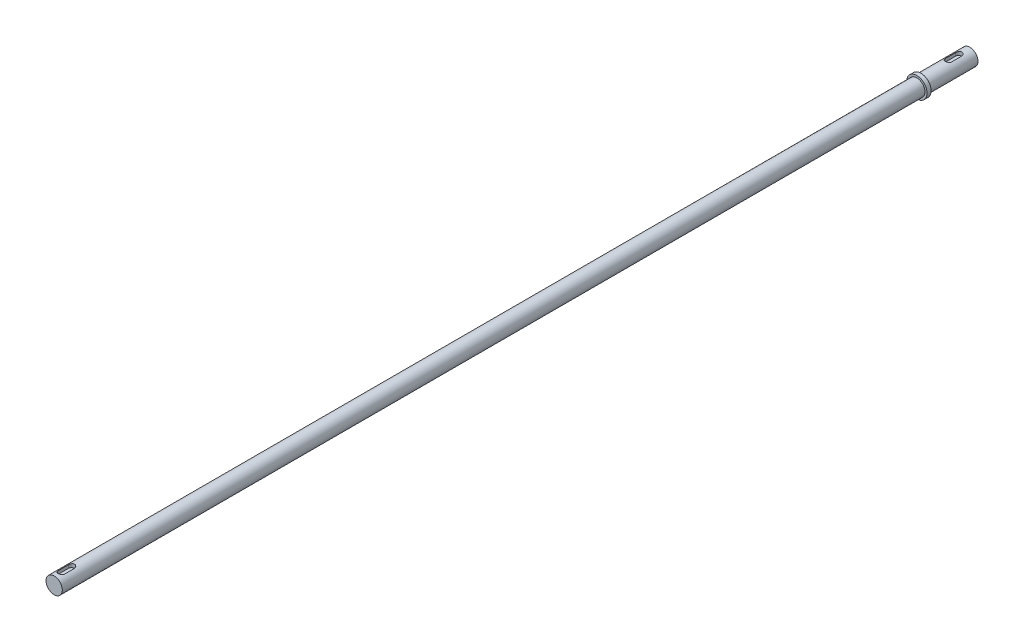
from build123d import *

# Parameters (mm, degrees)
SKETCH3_R           = 4
BOSS_EXTRUDE2_DEPTH = 14
SKETCH4_R           = 4
BOSS_EXTRUDE3_DEPTH = 10
SKETCH5_R           = 5
BOSS_EXTRUDE4_DEPTH = 2
CUT_EXTRUDE1_DEPTH  = 1.8
SKETCH7_R           = 4
BOSS_EXTRUDE5_DEPTH = 42
SKETCH8_R           = 4
BOSS_EXTRUDE7_DEPTH = 150
SKETCH9_R           = 4
BOSS_EXTRUDE8_DEPTH = 198
SKETCH10_R          = 4
BOSS_EXTRUDE9_DEPTH = 33.1
CUT_EXTRUDE2_DEPTH  = 1.8


with BuildPart() as part:
    # Sketch3 → Boss-Extrude2 (new body)
    with BuildSketch(Plane.XY):
        Circle(SKETCH3_R)
    extrude(amount=BOSS_EXTRUDE2_DEPTH)

    # Sketch4 → Boss-Extrude3 (add)
    with BuildSketch(Plane.XY.offset(14)):
        Circle(SKETCH4_R)
    extrude(amount=BOSS_EXTRUDE3_DEPTH)

    # Sketch5 → Boss-Extrude4 (add)
    with BuildSketch(Plane.XY.offset(24)):
        Circle(SKETCH5_R)
    extrude(amount=BOSS_EXTRUDE4_DEPTH)

    # Sketch6 → Cut-Extrude1 (cut)
    with BuildSketch(Plane(origin=(0, 4, 0), x_dir=(1, 0, 0), z_dir=(0, 1, 0))):
        with BuildLine():
            Line((1.5, -5.5), (1.5, -10.5))
            ThreePointArc((1.5, -10.5), (0, -12), (-1.5, -10.5))
            Line((-1.5, -10.5), (-1.5, -5.5))
            ThreePointArc((-1.5, -5.5), (0, -4), (1.5, -5.5))
        make_face()
    extrude(amount=-CUT_EXTRUDE1_DEPTH, mode=Mode.SUBTRACT)

    # Sketch7 → Boss-Extrude5 (add)
    with BuildSketch(Plane.XY.offset(26)):
        Circle(SKETCH7_R)
    extrude(amount=BOSS_EXTRUDE5_DEPTH)

    # Sketch8 → Boss-Extrude7 (add)
    with BuildSketch(Plane.XY.offset(68)):
        Circle(SKETCH8_R)
    extrude(amount=BOSS_EXTRUDE7_DEPTH)

    # Sketch9 → Boss-Extrude8 (add)
    with BuildSketch(Plane.XY.offset(218)):
        Circle(SKETCH9_R)
    extrude(amount=BOSS_EXTRUDE8_DEPTH)

    # Sketch10 → Boss-Extrude9 (add)
    with BuildSketch(Plane.XY.offset(416)):
        Circle(SKETCH10_R)
    extrude(amount=BOSS_EXTRUDE9_DEPTH)

    # Sketch13 → Cut-Extrude2 (cut)
    with BuildSketch(Plane(origin=(0, 4, 0), x_dir=(1, 0, 0), z_dir=(0, 1, 0))):
        with BuildLine():
            Line((1.5, -440.6), (1.5, -445.6))
            ThreePointArc((1.5, -445.6), (0, -447.1), (-1.5, -445.6))
            Line((-1.5, -445.6), (-1.5, -440.6))
            ThreePointArc((-1.5, -440.6), (0, -439.1), (1.5, -440.6))
        make_face()
    extrude(amount=-CUT_EXTRUDE2_DEPTH, mode=Mode.SUBTRACT)


solid = part.part
